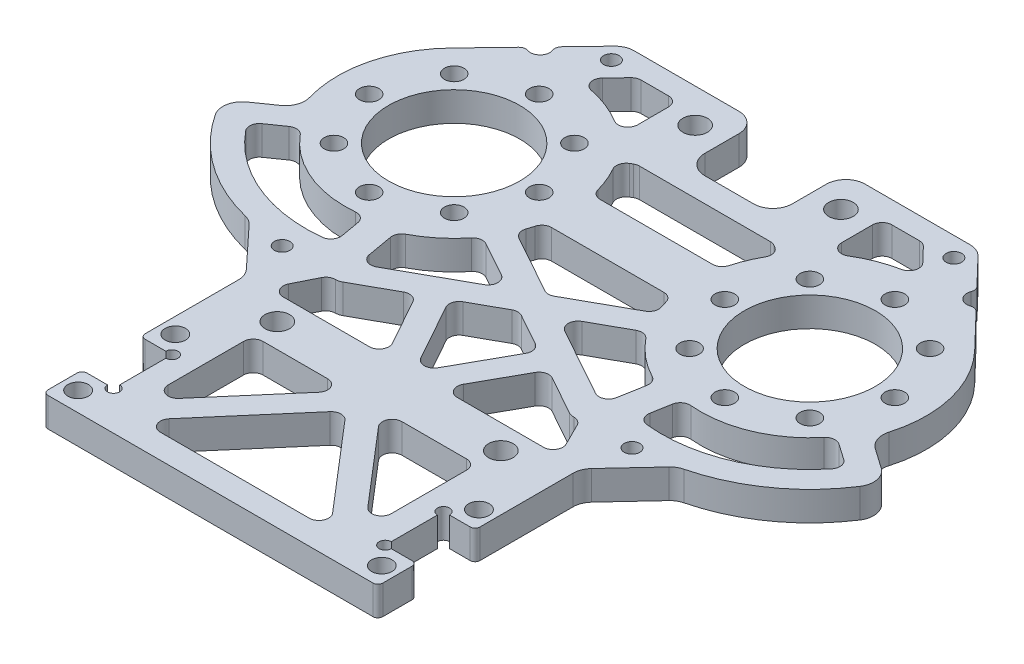
SolidWorks part; units mm, degrees
material "Thornel Mat VMA"
ref_plane "前视基准面" through (0, 0, 0) normal (0, 0, 1) x (1, 0, 0)
ref_plane "上视基准面" through (0, 0, 0) normal (0, 1, 0) x (1, 0, 0)
ref_plane "右视基准面" through (0, 0, 0) normal (1, 0, 0) x (0, 0, -1)
sketch "草图1" plane through (0, 0, 0) normal (0, 1, 0) x (1, 0, 0)
  line L0 (-15, 28) -> (15, 28) construction
  line L1 (-23, -50) -> (23, -50) construction
  line L2 (0, 28) -> (0, -50) construction
  line L3 (-36.6, 0) -> (36.6, 0) construction
  line L4 (-36.2611, 35) -> (-9, 35)
  line L5 (36.2611, 35) -> (53.9095, 16.6248)
  line L9 (-36.2611, 35) -> (-53.9095, 16.6248)
  line L11 (-34.45, -86.75) -> (34.45, -86.75)
  line L12 (34.45, -86.75) -> (34.45, -78.75)
  line L13 (-34.45, -66.75) -> (-29.2, -66.75)
  line L14 (-27.95, -68) -> (-27.95, -77.5)
  line L15 (-29.2, -78.75) -> (-34.45, -78.75)
  line L16 (-34.45, -78.75) -> (-34.45, -86.75)
  line L17 (27.95, -68) -> (27.95, -77.5)
  line L18 (34.45, -66.75) -> (29.2, -66.75)
  line L19 (29.2, -78.75) -> (34.45, -78.75)
  line L21 (-34.45, -66.75) -> (-34.45, -45)
  line L22 (34.45, -66.75) -> (34.45, -45)
  line L23 (-9, 35) -> (-9, 20)
  line L24 (9, 35) -> (9, 20)
  line L25 (-9, 20) -> (9, 20)
  line L26 (9, 35) -> (36.2611, 35)
  line L27 (-58.6962, -9.368) -> (-68.2579, -16.0632)
  line L28 (-55.0309, -12.9055) -> (-61.5841, -17.4941)
  line L29 (-32.6929, -22.1582) -> (-31.3037, -30.0366)
  line L30 (55.0309, -12.9055) -> (61.5841, -17.4941)
  line L31 (-36.6, 0) -> (-48.9744, -12.3744) construction
  line L32 (-36.6, 0) -> (-36.6, -17.5) construction
  line L33 (32.6929, -22.1582) -> (31.3037, -30.0366)
  line L34 (58.6962, -9.368) -> (68.2579, -16.0632)
  line L35 (-34.45, -45) -> (-44.0313, -34.7135)
  line L36 (34.45, -45) -> (44.0313, -34.7135)
  line L37 (36, -36) -> (-36, -36) construction
  circle A0 centre (-36.6, 0) radius 13.5
  circle A2 centre (-15, 28) radius 2.525
  circle A3 centre (15, 28) radius 2.525
  circle A4 centre (-23, -50) radius 2.525
  circle A5 centre (23, -50) radius 2.525
  circle A6 centre (-36.6, 0) radius 17.5 construction
  circle A7 centre (36.6, 0) radius 13.5
  circle A8 centre (36.6, 0) radius 17.5 construction
  circle A9 centre (-36.6, 17.5) radius 2.01
  circle A10 centre (-24.2256, 12.3744) radius 2.01
  circle A11 centre (-19.1, 0) radius 2.01
  circle A12 centre (-24.2256, -12.3744) radius 2.01
  circle A13 centre (-36.6, -17.5) radius 2.01
  circle A14 centre (-48.9744, -12.3744) radius 2.01
  circle A15 centre (-54.1, 0) radius 2.01
  circle A16 centre (-48.9744, 12.3744) radius 2.01
  circle A17 centre (48.9744, 12.3744) radius 2.01
  circle A18 centre (54.1, 0) radius 2.01
  circle A19 centre (48.9744, -12.3744) radius 2.01
  circle A20 centre (36.6, -17.5) radius 2.01
  circle A21 centre (24.2256, -12.3744) radius 2.01
  circle A22 centre (19.1, 0) radius 2.01
  circle A23 centre (24.2256, 12.3744) radius 2.01
  circle A24 centre (36.6, 17.5) radius 2.01
  arc A25 (-53.9095, 16.6248) -> (-58.6962, -9.368) centre (-36.6, 0) ccw
  arc A26 (53.9095, 16.6248) -> (58.6962, -9.368) centre (36.6, 0) cw
  arc A31 (-27.95, -68) -> (-29.2, -66.75) centre (-27.95, -66.75) ccw
  arc A32 (-29.2, -78.75) -> (-27.95, -77.5) centre (-27.95, -78.75) ccw
  arc A33 (29.2, -78.75) -> (27.95, -77.5) centre (27.95, -78.75) cw
  arc A34 (27.95, -68) -> (29.2, -66.75) centre (27.95, -66.75) cw
  circle A35 centre (-31.25, -82.75) radius 2.1
  circle A36 centre (-31.25, -62.75) radius 2.1
  circle A37 centre (31.25, -82.75) radius 2.1
  circle A38 centre (31.25, -62.75) radius 2.1
  circle A39 centre (-35.25, 31) radius 1.6
  circle A40 centre (35.25, 31) radius 1.6
  circle A42 centre (-15, 28) radius 7 construction
  circle A43 centre (15, 28) radius 7 construction
  arc A44 (-61.5841, -17.4941) -> (-31.3037, -30.0366) centre (-36.6, 0) ccw
  arc A45 (-68.2579, -16.0632) -> (-44.0313, -34.7135) centre (-36.6, 0) ccw
  arc A46 (-55.0309, -12.9055) -> (-32.6929, -22.1582) centre (-36.6, 0) ccw
  arc A47 (55.0309, -12.9055) -> (32.6929, -22.1582) centre (36.6, 0) cw
  arc A48 (61.5841, -17.4941) -> (31.3037, -30.0366) centre (36.6, 0) cw
  arc A49 (68.2579, -16.0632) -> (44.0313, -34.7135) centre (36.6, 0) cw
  circle A50 centre (-36, -36) radius 1.6
  circle A51 centre (36, -36) radius 1.6
  point P36 (-36.6, 0)
  dimension "D1" = 27
  dimension "D2" = 30
  dimension "D6" = 35
  dimension "D8" = 5.05
  dimension "D9" = 8
  dimension "D10" = 4.02
  dimension "D11" = 3.2
  dimension "D13" = 8
  dimension "D15" = 24
  dimension "D16" = 1.25
  dimension "D19" = 4.2
  dimension "D23" = 3.2
  dimension "D30" = 10
  dimension "D31" = 5
  dimension "D34" = 22.5
  dimension "D35" = 3.2
  dimension "D3" = 46
  dimension "D4" = 78
  dimension "D5" = 28
  dimension "D7" = 73.2
  dimension "D12" = 20
  dimension "D14" = 62.5
  dimension "D17" = 3.3
  dimension "D18" = 12
  dimension "D20" = 4
  dimension "D21" = 4
  dimension "D22" = 12.75
  dimension "D24" = 3
  dimension "D25" = 70.5
  dimension "D26" = 7
  dimension "D27" = 3.5
  dimension "D28" = 18
  dimension "D29" = 8
  dimension "D32" = 5
  dimension "D33" = 10
  dimension "D36" = 36
  dimension "D37" = 72
  dimension "D38" = 5
  dimension "D39" = 5
extrude "凸台-拉伸1" add sketch "草图1" along normal blind 6
sketch "草图3" plane through (0, 6, 0) normal (0, 1, 0) x (1, 0, 0)
  line L0 (0, 35) -> (0, -86.75) construction
  line L1 (-35.7483, 23.9849) -> (-29.4909, 30.5)
  line L2 (-34.45, -86.75) -> (34.45, -86.75) construction
  line L3 (-36.6, 0) -> (36.6, 0) construction
  line L4 (-13.1266, 5) -> (13.1266, 5)
  line L5 (-13.1266, -5) -> (13.1266, -5)
  line L6 (-16.7122, 13.4341) -> (-14, 15)
  line L7 (16.7122, 13.4341) -> (14, 15)
  line L8 (-14, 15) -> (14, 15)
  line L9 (-26.6559, -21.843) -> (-24.5123, -34)
  line L10 (26.6559, -21.843) -> (24.5123, -34)
  line L11 (-30, -45) -> (30, -45)
  line L12 (-15, 28) -> (15, 28) construction
  line L13 (-23, -50) -> (23, -50) construction
  line L14 (-27.95, -68) -> (-27.95, -77.5) construction
  line L15 (19.656, -81.75) -> (-19.656, -81.75)
  line L16 (22.95, -77.9106) -> (22.95, -55)
  line L17 (22.95, -55) -> (3.294, -55)
  line L18 (-22.95, -77.9106) -> (-22.95, -55)
  line L19 (22.95, -81.75) -> (-22.95, -55) construction
  line L20 (22.95, -55) -> (-22.95, -81.75) construction
  line L21 (-22.95, -81.75) -> (0, -55) construction
  line L22 (0, -55) -> (22.95, -81.75) construction
  line L23 (-3.294, -55) -> (-22.95, -77.9106)
  line L24 (0, -58.8394) -> (-19.656, -81.75)
  line L25 (0, -58.8394) -> (19.656, -81.75)
  line L26 (3.294, -55) -> (22.95, -77.9106)
  line L27 (-3.294, -55) -> (-22.95, -55)
  line L28 (-9, 35) -> (-36.2611, 35) construction
  line L29 (-24.5123, -34) -> (-30, -45)
  line L30 (24.5123, -34) -> (30, -45)
  line L31 (-31.3037, -30.0366) -> (-32.6929, -22.1582) construction
  line L32 (-24.5123, -34) -> (15.6273, -11.6682) construction
  line L33 (-25.7278, -31.8153) -> (14.4119, -9.4835)
  line L34 (-23.2969, -36.1847) -> (16.8428, -13.8529)
  line L35 (24.5123, -34) -> (-15.6273, -11.6682) construction
  line L36 (25.7278, -31.8153) -> (-14.4119, -9.4835)
  line L37 (23.2969, -36.1847) -> (-16.8428, -13.8529)
  line L38 (0, -50) -> (-12.5915, -27.3678) construction
  line L39 (-2.1847, -51.2154) -> (-14.7761, -28.5832)
  line L40 (2.1847, -48.7846) -> (-10.4068, -26.1524)
  line L41 (0, -50) -> (12.5915, -27.3678) construction
  line L42 (2.1847, -51.2154) -> (14.7761, -28.5832)
  line L43 (-2.1847, -48.7846) -> (10.4068, -26.1524)
  line L44 (-29.4909, 30.5) -> (-21, 30.5)
  line L45 (-21, 30.5) -> (-21, 18.2384)
  line L46 (-36.2611, 35) -> (-53.9095, 16.6248) construction
  line L47 (29.4909, 30.5) -> (21, 30.5)
  line L48 (35.7483, 23.9849) -> (29.4909, 30.5)
  line L49 (21, 30.5) -> (21, 18.2384)
  arc A0 (-13.1266, 5) -> (-16.7122, 13.4341) centre (-36.6, 0) ccw
  arc A1 (13.1266, 5) -> (16.7122, 13.4341) centre (36.6, 0) cw
  arc A2 (-53.9095, 16.6248) -> (-58.6962, -9.368) centre (-36.6, 0) ccw construction
  arc A3 (-26.6559, -21.843) -> (-13.1266, -5) centre (-36.6, 0) ccw
  arc A4 (26.6559, -21.843) -> (13.1266, -5) centre (36.6, 0) cw
  arc A5 (-25.7278, -31.8153) -> (-23.2969, -36.1847) centre (-24.5123, -34) ccw
  arc A6 (16.8428, -13.8529) -> (14.4119, -9.4835) centre (15.6273, -11.6682) ccw
  arc A7 (25.7278, -31.8153) -> (23.2969, -36.1847) centre (24.5123, -34) cw
  arc A8 (-16.8428, -13.8529) -> (-14.4119, -9.4835) centre (-15.6273, -11.6682) cw
  arc A9 (-2.1847, -51.2154) -> (2.1847, -48.7846) centre (0, -50) ccw
  arc A10 (-10.4068, -26.1524) -> (-14.7761, -28.5832) centre (-12.5915, -27.3678) ccw
  arc A11 (2.1847, -51.2154) -> (-2.1847, -48.7846) centre (0, -50) cw
  arc A12 (10.4068, -26.1524) -> (14.7761, -28.5832) centre (12.5915, -27.3678) cw
  arc A13 (-35.7483, 23.9849) -> (-21, 18.2384) centre (-36.6, 0) cw
  arc A14 (35.7483, 23.9849) -> (21, 18.2384) centre (36.6, 0) ccw
  point P35 (0, -68.375)
  point P51 (-4.4425, -22.8341)
  point P58 (4.4425, -22.8341)
  point P65 (-6.2957, -38.6839)
  point P72 (6.2957, -38.6839)
  dimension "D1" = 10
  dimension "D14" = 8
  dimension "D2" = 13
  dimension "D3" = 150
  dimension "D4" = 28
  dimension "D5" = 5
  dimension "D6" = 6
  dimension "D7" = 5
  dimension "D8" = 5
  dimension "D9" = 5
  dimension "D10" = 5
  dimension "D11" = 5
  dimension "D12" = 60
  dimension "D13" = 11
  dimension "D15" = 4.5
  dimension "D16" = 6
extrude "切除-拉伸1" cut sketch "草图3" against normal through all contours L1 A13 L45 L44 | A14 L48 L47 L49 | L4 A1 L7 L8 L6 A0 | A3 A8 L36 L33 A6 A4 L5 | L37 A8 A3 L9 L33 | A5 L29 L11 L39 L34 | L40 L43 L37 L34 | A6 L34 L36 L10 A4 | L30 A7 L37 L42 L11 | L23 L27 L18 | L25 L24 L15 | L17 L26 L16
fillet "R2 镂空圆角" radius 2 56 edges at (-13.1266, 3, 5) (13.1266, 3, 5) (26.6559, 3, 21.843) (-26.6559, 3, 21.843) (22.95, 3, 55) (22.95, 3, 77.9106) (3.294, 3, 55) (19.656, 3, 81.75) (-19.656, 3, 81.75) (0, 3, 58.8394) (-3.294, 3, 55) (-22.95, 3, 77.9106) (-22.95, 3, 55) (-16.7122, 3, -13.4341) (14, 3, -15) (16.7122, 3, -13.4341) (13.1266, 3, -5) (-13.1266, 3, -5) (-14, 3, -15) (21, 3, -30.5) (29.4909, 3, -30.5) (35.7483, 3, -23.9849) (21, 3, -18.2384) (-5.1422, 3, 20.3625) (-24.9717, 3, 31.3947) (-16.9549, 3, 13.7866) (-14.5273, 3, 9.4232) (14.5273, 3, 9.4232) (16.9549, 3, 13.7866) (0, 3, 17.5016) (24.9717, 3, 31.3947) (5.1422, 3, 20.3625) (5.6426, 3, 45) (13.5607, 3, 30.7679) (25.6284, 3, 36.2371) (30, 3, 45) (-13.5607, 3, 30.7679) (-5.6426, 3, 45) (-30, 3, 45) (-25.6284, 3, 36.2371) (0, 3, 23.2234) (9.1914, 3, 28.337) (0, 3, 44.8578) (-9.1914, 3, 28.337) (-21, 3, -30.5) (-21, 3, -18.2384) (-35.7483, 3, -23.9849) (61.5841, 3, 17.4941) (31.3037, 3, 30.0366) (32.6929, 3, 22.1582) (55.0309, 3, 12.9055) (-31.3037, 3, 30.0366) (-61.5841, 3, 17.4941) (-55.0309, 3, 12.9055) (-32.6929, 3, 22.1582) (-29.4909, 3, -30.5)
fillet "R1 插接圆角" radius 1 6 edges at (34.45, 3, 66.75) (34.45, 3, 78.75) (34.45, 3, 86.75) (-34.45, 3, 86.75) (-34.45, 3, 78.75) (-34.45, 3, 66.75)
fillet "R4 外缘圆角" radius 4 14 edges at (34.45, 3, 45) (44.0313, 3, 34.7135) (68.2579, 3, 16.0632) (58.6962, 3, 9.368) (-34.45, 3, 45) (-44.0313, 3, 34.7135) (-68.2579, 3, 16.0632) (-58.6962, 3, 9.368) (36.2611, 3, -35) (9, 3, -35) (9, 3, -20) (-9, 3, -20) (-9, 3, -35) (-36.2611, 3, -35)
sketch "草图4" plane through (0, 6, 0) normal (0, 1, 0) x (1, 0, 0)
  line L0 (-37.4416, 33.7708) -> (-53.9095, 16.6248) construction
  line L1 (-42.7146, 28.2807) -> (-47.0956, 23.7193)
  line L2 (0, 20) -> (0, 0) construction
  line L3 (5, 20) -> (-5, 20) construction
  line L4 (42.7146, 28.2807) -> (47.0956, 23.7193)
  arc A0 (-45.5386, 24.103) -> (-43.0351, 26.7095) centre (-44.9051, 26) ccw
  arc A1 (-45.5386, 24.103) -> (-47.0956, 23.7193) centre (-46.0137, 22.6802) ccw
  arc A2 (-42.7146, 28.2807) -> (-43.0351, 26.7095) centre (-41.6327, 27.2417) ccw
  arc A3 (45.5386, 24.103) -> (47.0956, 23.7193) centre (46.0137, 22.6802) cw
  arc A4 (42.7146, 28.2807) -> (43.0351, 26.7095) centre (41.6327, 27.2417) cw
  arc A5 (45.5386, 24.103) -> (43.0351, 26.7095) centre (44.9051, 26) cw
  point P21 (-44.7133, 26.1997)
  dimension "D1" = 2
  dimension "D2" = 1.5
  dimension "D3" = 26
extrude "73.20标识" cut sketch "草图4" against normal through all
